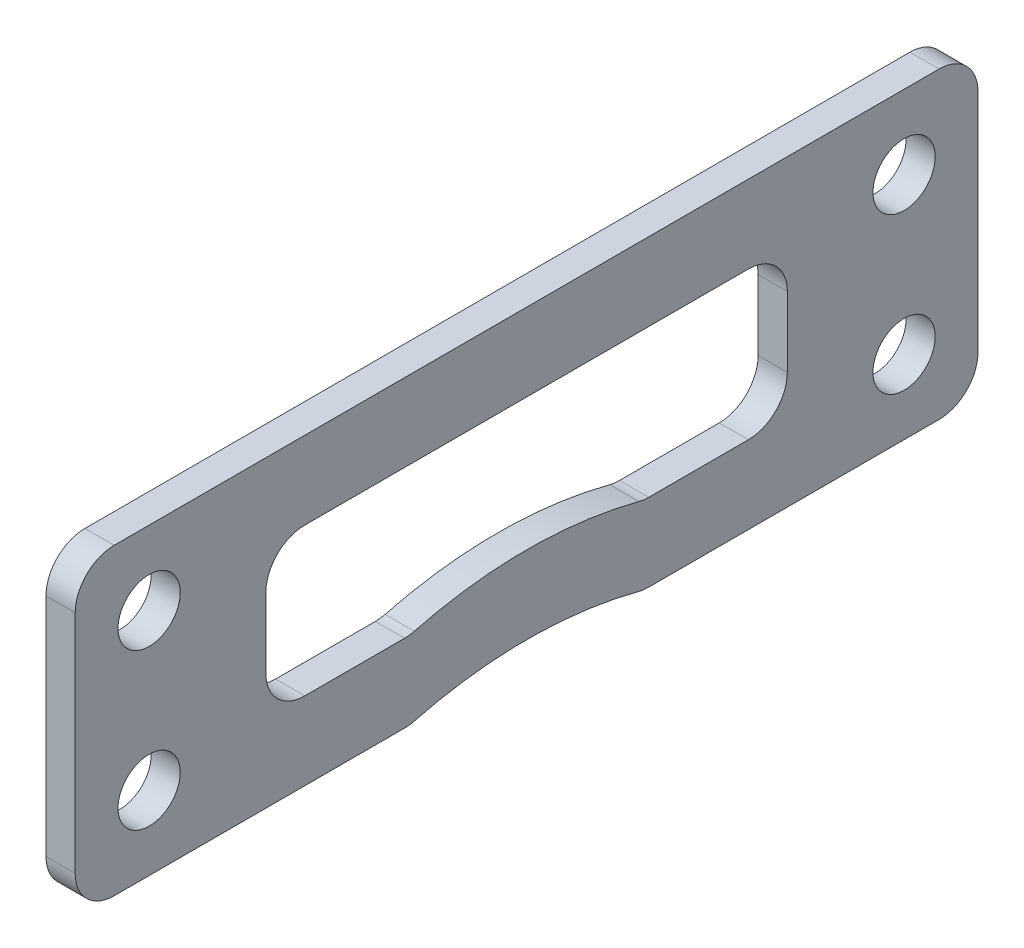
from build123d import *

# Parameters (mm, degrees)
SKETCH_1_W          = 46.4
SKETCH_1_H          = 15.6
SKETCH_1_R          = 1.6
EXTRUDE_1_DEPTH     = 1.5
SKETCH_2_R          = 23
CUT_EXTRUDE_1_DEPTH = 45.229515032
CUT_EXTRUDE_2_DEPTH = 45.229515032
FILLET_1_R          = 2


with BuildPart() as part:
    # 草图1 → 凸台-拉伸1 (new body)
    with BuildSketch(Plane(origin=(0, 0, 0), x_dir=(0, 0, -1), z_dir=(1, 0, 0))):
        with Locations((19.4, -4)):
            Rectangle(SKETCH_1_W, SKETCH_1_H)
        Circle(SKETCH_1_R, mode=Mode.SUBTRACT)
        with Locations((0, -8)):
            Circle(SKETCH_1_R, mode=Mode.SUBTRACT)
        with Locations((38.8, 0)):
            Circle(SKETCH_1_R, mode=Mode.SUBTRACT)
        with Locations((38.8, -8)):
            Circle(SKETCH_1_R, mode=Mode.SUBTRACT)
    extrude(amount=EXTRUDE_1_DEPTH)

    # 草图2 → 切除-拉伸1 (cut, through all)
    with BuildSketch(Plane(origin=(1.5, 0, 0), x_dir=(0, 0, -1), z_dir=(1, 0, 0))):
        with Locations((19.4, -34)):
            Circle(SKETCH_2_R)
    extrude(amount=-CUT_EXTRUDE_1_DEPTH, mode=Mode.SUBTRACT)

    # 草图3 → 切除-拉伸2 (cut, through all)
    with BuildSketch(Plane(origin=(1.5, 0, 0), x_dir=(0, 0, -1), z_dir=(1, 0, 0))):
        with BuildLine():
            Line((6, -0.2), (32.8, -0.2))
            Line((32.8, -0.2), (32.8, -7.8))
            Line((32.8, -7.8), (25.413318551, -7.8))
            ThreePointArc((25.413318551, -7.8), (19.4, -7), (13.386681449, -7.8))
            Line((13.386681449, -7.8), (6, -7.8))
            Line((6, -7.8), (6, -0.2))
        make_face()
    extrude(amount=-CUT_EXTRUDE_2_DEPTH, mode=Mode.SUBTRACT)

    # 圆角1
    fillet_1_edges = [part.edges().sort_by_distance(p)[0] for p in [
        (0.75, -11.8, -25.413318551),
        (0.75, -11.8, -13.386681449),
        (0.75, -7.8, -6),
        (0.75, -0.2, -6),
        (0.75, -0.2, -32.8),
        (0.75, -7.8, -32.8),
        (0.75, -7.8, -25.413318551),
        (0.75, -7.8, -13.386681449),
        (0.75, 3.8, 3.8),
        (0.75, 3.8, -42.6),
        (0.75, -11.8, -42.6),
        (0.75, -11.8, 3.8),
    ]]
    fillet(fillet_1_edges, radius=FILLET_1_R)


solid = part.part
